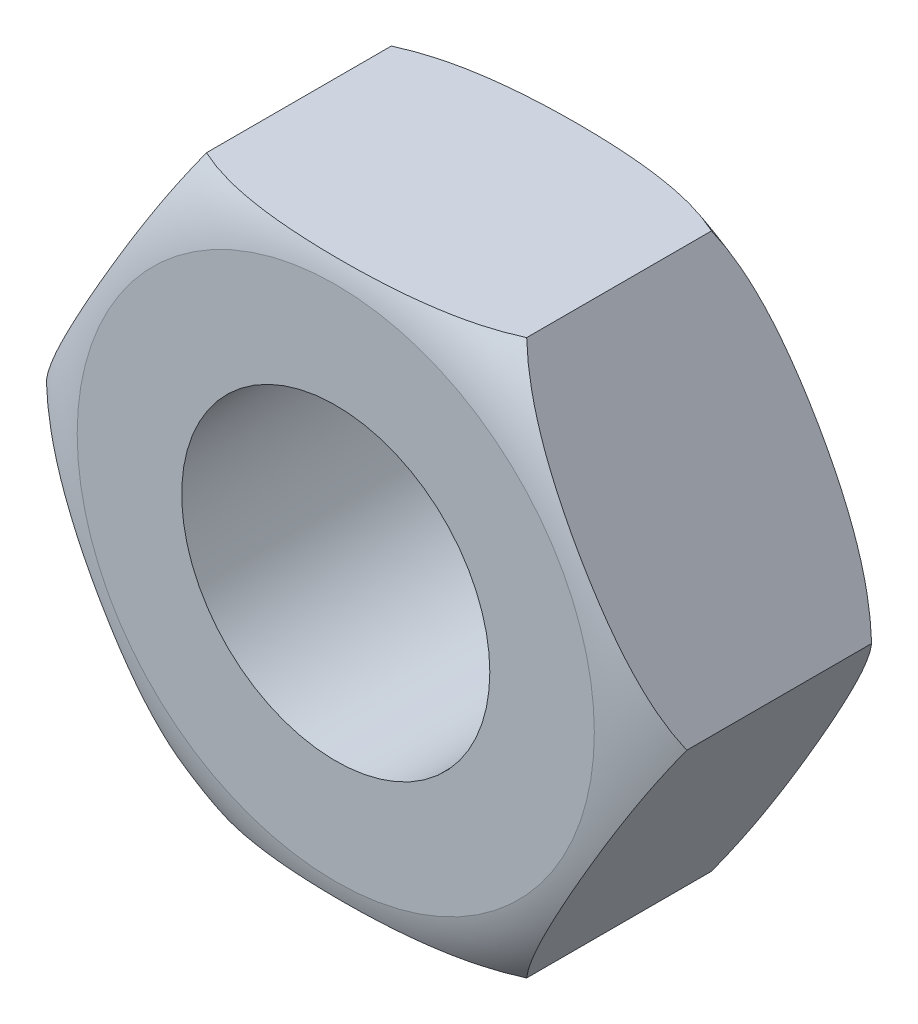
SolidWorks part; units mm, degrees
ref_plane "Front" through (0, 0, 0) normal (0, 0, 1) x (1, 0, 0)
ref_plane "Top" through (0, 0, 0) normal (0, 1, 0) x (1, 0, 0)
ref_plane "Right" through (0, 0, 0) normal (1, 0, 0) x (0, 0, -1)
sketch "Sketch5" plane through (0, 0, 0) normal (0, 0, 1) x (1, 0, 0)
  line L1 (10.3923, 0) -> (5.1962, 9)
  line L2 (5.1962, 9) -> (-5.1962, 9)
  line L3 (-5.1962, 9) -> (-10.3923, 0)
  line L4 (-10.3923, 0) -> (-5.1962, -9)
  line L5 (-5.1962, -9) -> (5.1962, -9)
  line L6 (5.1962, -9) -> (10.3923, 0)
  circle A0 centre (0, 0) radius 9 construction
  circle A1 centre (0, 0) radius 5
  dimension "D2" = 10
  dimension "D1" = 18
extrude "Boss-Extrude2" add sketch "Sketch5" along normal blind 8
sketch "Sketch6" plane through (0, 0, 0) normal (0, 1, 0) x (1, 0, 0)
  line L0 (-10.3923, 0) -> (-10.3923, -1)
  line L1 (-10.3923, -8) -> (-10.3923, 0) construction
  line L2 (-10.3923, 0) -> (-8.3923, 0)
  line L3 (-5.1962, 0) -> (-10.3923, 0) construction
  line L6 (0, 0) -> (0, -8.2405) construction
  line L7 (-10.3923, -8) -> (-8.3923, -8)
  line L8 (-10.3923, -8) -> (-10.3923, -7)
  arc A0 (-10.3923, -1) -> (-8.3923, 0) centre (-7.6747, -3.9351) cw
  arc A1 (-10.3923, -7) -> (-8.3923, -8) centre (-7.6747, -4.0649) ccw
  dimension "D3" = 4
  dimension "D1" = 1
  dimension "D2" = 2
revolve "Cut-Revolve2" cut sketch "Sketch6" angle 360 about L6
scale "Scale 1" bodies to scale 104 scale about centroid uniform scaling yes scale factor 1.875
